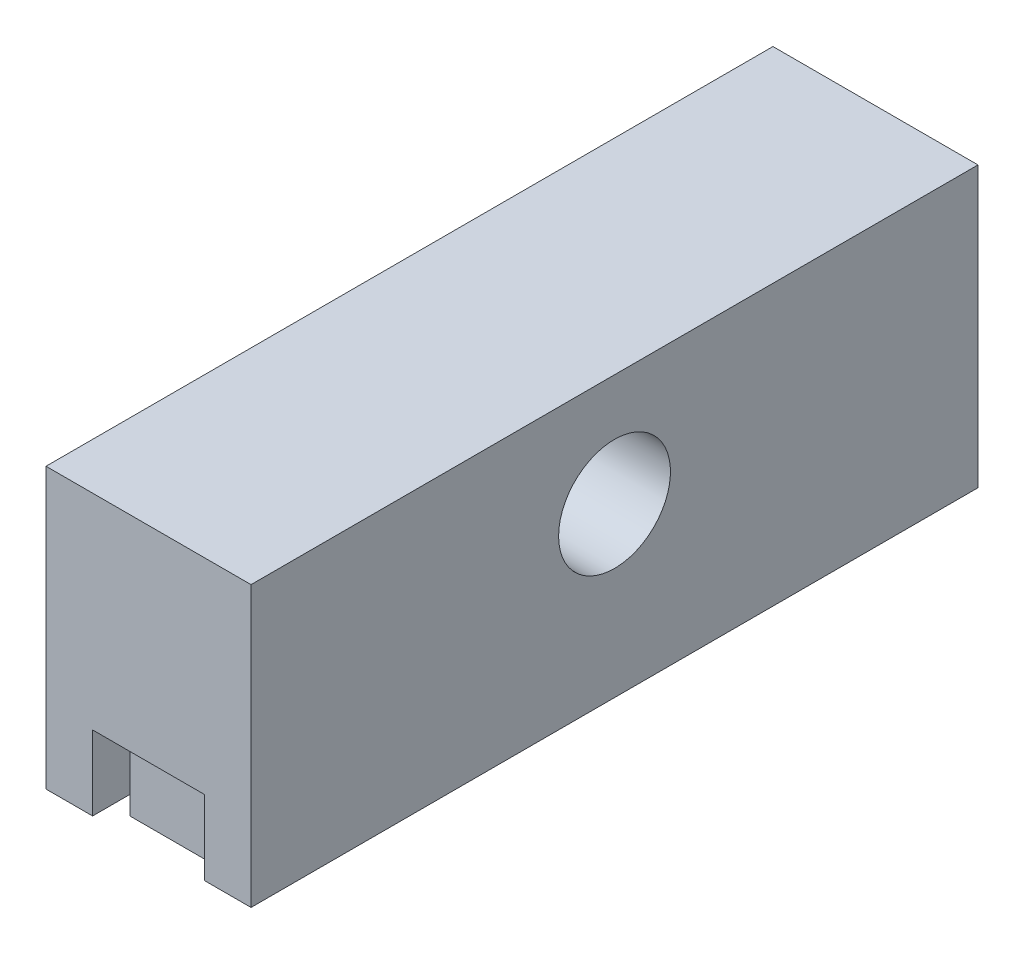
SolidWorks part; units mm, degrees
ref_plane "前视基准面" through (0, 0, 0) normal (0, 0, 1) x (1, 0, 0)
ref_plane "上视基准面" through (0, 0, 0) normal (0, 1, 0) x (1, 0, 0)
ref_plane "右视基准面" through (0, 0, 0) normal (1, 0, 0) x (0, 0, -1)
other "Configuration Table"
sketch "草图1" plane through (0, 0, 0) normal (0, 0, 1) x (1, 0, 0)
  line L0 (3, -7.5) -> (5.5, -7.5)
  line L1 (-5.5, -7.5) -> (-3, -7.5)
  line L2 (-5.5, -7.5) -> (-5.5, 7.5)
  line L3 (-5.5, 7.5) -> (5.5, 7.5)
  line L4 (5.5, -7.5) -> (5.5, 7.5)
  line L5 (0, 7.5) -> (0, -10.0626) construction
  line L6 (-5.5, 0) -> (5.5, 0) construction
  line L8 (-3, -7.5) -> (-3, -3.5)
  line L9 (-3, -3.5) -> (3, -3.5)
  line L10 (3, -7.5) -> (3, -3.5)
  point P0 (0, 0)
  dimension "D1" = 4
  dimension "D2" = 6
  dimension "D3" = 15
  dimension "D4" = 11
  dimension "D5" = 3
extrude "凸台-拉伸1" add sketch "草图1" along normal mid plane 39
sketch "草图2" plane through (0, -3.5, 0) normal (0, -1, 0) x (1, 0, 0)
  line L0 (3, 19.5) -> (3, -19.5) construction
  line L1 (-3, -17.5) -> (3, -17.5)
  line L2 (-3, -17.5) -> (-3, 17.5)
  line L3 (-3, 17.5) -> (3, 17.5)
  line L5 (3, -17.5) -> (3, 17.5)
  line L7 (0, 17.5) -> (0, -17.5) construction
  line L12 (-3, 0) -> (3, 0) construction
  point P0 (0, 0)
  dimension "D1" = 35
extrude "凸台-拉伸2" add sketch "草图2" along normal blind 5 separate body
sketch "草图3" plane through (-5.5, 0, 0) normal (-1, 0, 0) x (0, 0, 1)
  line L0 (17.5, -8.5) -> (-17.5, -8.5) construction
  line L1 (-19.5, 7.5) -> (-19.5, -7.5) construction
  circle A0 centre (0, 1.5) radius 3
  dimension "D3" = 6
  dimension "D1" = 10
  dimension "D2" = 19.5
extrude "切除-拉伸1" cut sketch "草图3" against normal up to next (11 mm away)
